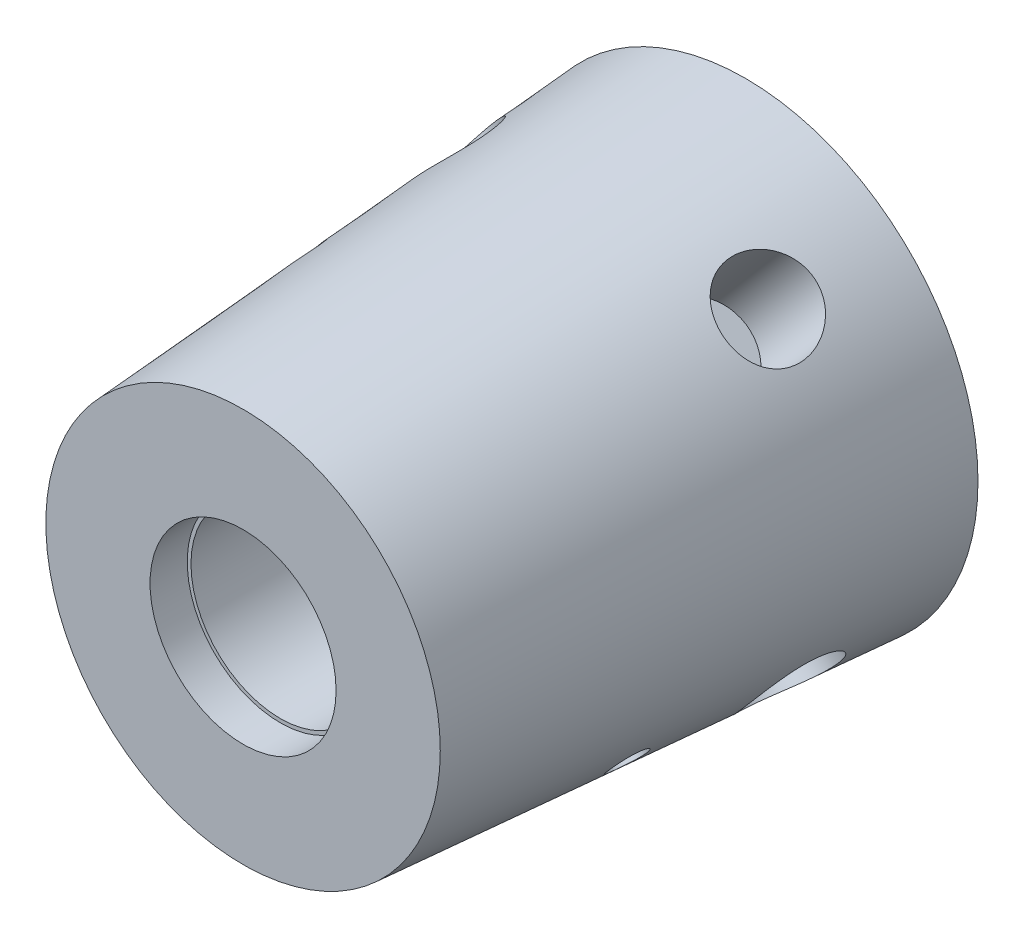
from build123d import *

# Parameters (mm, degrees)
F_10_0_10_DIAMETER_HOLE1_D        = 10
F_10_0_10_DIAMETER_HOLE1_DEPTH    = 22.574074074
F_10_0_10_DIAMETER_HOLE2_D        = 10
F_10_0_10_DIAMETER_HOLE2_DEPTH    = 22.574074074
F_24_0_24_DIAMETER_HOLE1_D        = 24
F_24_0_24_DIAMETER_HOLE1_DEPTH    = 27.01345843
F_24_0_24_DIAMETER_HOLE2_D        = 24
F_24_0_24_DIAMETER_HOLE2_DEPTH    = 27.01345843
F_24_0_24_DIAMETER_HOLE3_D        = 24
F_24_0_24_DIAMETER_HOLE3_DEPTH    = 27.01345843
F_24_0_24_DIAMETER_HOLE4_D        = 24
F_24_0_24_DIAMETER_HOLE4_DEPTH    = 27.01345843
M42_COUNTERBORE_HOLE1_D           = 48
M42_COUNTERBORE_HOLE1_CBORE_D     = 50
M42_COUNTERBORE_HOLE1_CBORE_DEPTH = 10


with BuildPart() as part:
    # Sketch1 → Revolve1 (revolve)
    with BuildSketch(Plane(origin=(0, 234.743963655, 0), x_dir=(1, 0, 0), z_dir=(0, 1, 0))):
        Polygon((583.730642584, 1284.998443067), (521.230642584, 1284.998443067), (521.230642584, 1149.998443067), (574.230642584, 1149.998443067), align=None)
    revolve(axis=Axis((521.230642584, 234.743963655, -1284.998443067), (0, 0, 1)))

    # Ø10.0 (10) diameter hole1
    with Locations(Plane(origin=(137.830540227, -119.518291539, 0), x_dir=(0, 0, 1), z_dir=(-0.7555122914421019, 0.6551344728221105, -4.1215083496546135e-15))):
        with Locations((-1209.998443067, 518.828112131)):
            Hole(F_10_0_10_DIAMETER_HOLE1_D / 2, depth=F_10_0_10_DIAMETER_HOLE1_DEPTH)

    # Ø10.0 (10) diameter hole2
    with Locations(Plane(origin=(224.826381489, -194.955812873, 0), x_dir=(0, 0, -1), z_dir=(0.7555122914421021, -0.6551344728221103, 4.1124165324552015e-15))):
        with Locations((1209.998443067, 518.828112131)):
            Hole(F_10_0_10_DIAMETER_HOLE2_D / 2, depth=F_10_0_10_DIAMETER_HOLE2_DEPTH)

    # Ø24.0 (24) diameter hole1
    with Locations(Plane(origin=(135.232043071, -117.265032283, 0), x_dir=(0, 0, 1), z_dir=(-0.7555122914421021, 0.6551344728221103, 2.8630302475456504e-15))):
        with Locations((-1251.873904967, 518.828112131)):
            Hole(F_24_0_24_DIAMETER_HOLE1_D / 2, depth=F_24_0_24_DIAMETER_HOLE1_DEPTH)

    # Ø24.0 (24) diameter hole2
    with Locations(Plane(origin=(299.930161803, 345.884598073, 0), x_dir=(-0.7555122914421089, 0.6551344728221025, -3.5502706463705578e-15), z_dir=(-0.6551344728221025, -0.755512291442109, 4.094232898056383e-15))):
        with Locations((-240.007294272, 1251.873904967)):
            Hole(F_24_0_24_DIAMETER_HOLE2_D / 2, depth=F_24_0_24_DIAMETER_HOLE2_DEPTH)

    # Ø24.0 (24) diameter hole3
    with Locations(Plane(origin=(379.87420165, 438.077433648, 0), x_dir=(0.7555122914421041, -0.6551344728221079, -2.4905301953140895e-15), z_dir=(0.6551344728221079, 0.7555122914421041, 2.87212206474506e-15))):
        with Locations((240.007294272, 1251.873904967)):
            Hole(F_24_0_24_DIAMETER_HOLE3_D / 2, depth=F_24_0_24_DIAMETER_HOLE3_DEPTH)

    # Ø24.0 (24) diameter hole4
    with Locations(Plane(origin=(227.424878645, -197.20907213, 0), x_dir=(0, 0, -1), z_dir=(0.7555122914421021, -0.6551344728221103, 4.1124165324552015e-15))):
        with Locations((1251.873904967, 518.828112131)):
            Hole(F_24_0_24_DIAMETER_HOLE4_D / 2, depth=F_24_0_24_DIAMETER_HOLE4_DEPTH)

    # M42 counterbore hole1 (through all)
    with Locations(Plane.XY.offset(-1149.998443067)):
        with Locations((521.230642584, 234.743963655)):
            CounterBoreHole(M42_COUNTERBORE_HOLE1_D / 2, M42_COUNTERBORE_HOLE1_CBORE_D / 2, M42_COUNTERBORE_HOLE1_CBORE_DEPTH)


solid = part.part
